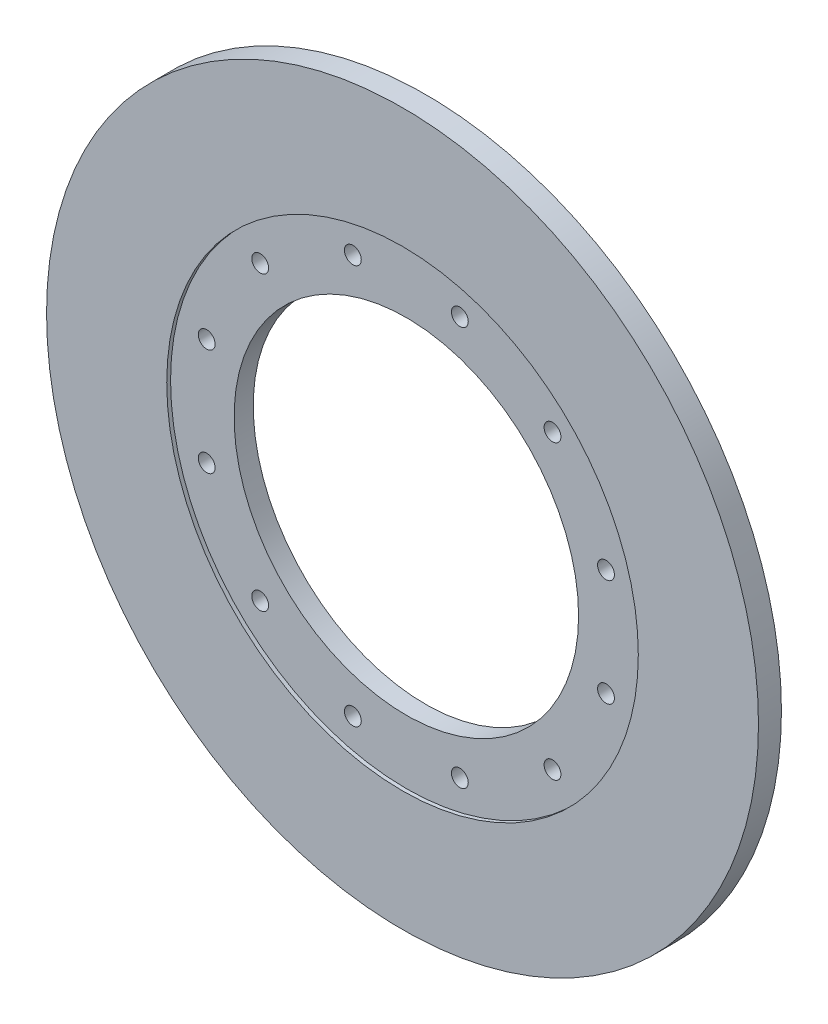
from build123d import *

# Parameters (mm, degrees)
SKETCH1_R               = 465
SKETCH1_R_2             = 225
BOSS_EXTRUDE1_DEPTH     = 30
SKETCH2_R               = 308
CUT_EXTRUDE1_DEPTH      = 5
CUT_EXTRUDE7_DEPTH      = 659.293247725
CUT_EXTRUDE7_DEPTH_BACK = 659.293247725
SKETCH4_R               = 11


with BuildPart() as part:
    # Sketch1 → Boss-Extrude1 (new body)
    with BuildSketch(Plane.XY):
        Circle(SKETCH1_R)
        Circle(SKETCH1_R_2, mode=Mode.SUBTRACT)
    extrude(amount=BOSS_EXTRUDE1_DEPTH)

    # Sketch2 → Cut-Extrude1 (cut)
    with BuildSketch(Plane.XY.offset(30)):
        Circle(SKETCH2_R)
    extrude(amount=-CUT_EXTRUDE1_DEPTH, mode=Mode.SUBTRACT)

    # Sketch4 → Cut-Extrude7 (cut, two sides: drawn at the far end of the back side and taken through both)
    with BuildSketch(Plane(origin=(0, 0, 0), x_dir=(-1, 0, 0), z_dir=(0, 0, -1)).offset(-CUT_EXTRUDE7_DEPTH_BACK)):
        with Locations(Location((-260.799973098, 69.881142178, 0), (0, 0, 180))):
            Circle(SKETCH4_R)
        with Locations(Location((-190.91883092, 190.91883092, 0), (0, 0, 180))):
            Circle(SKETCH4_R)
        with Locations(Location((-69.881142178, 260.799973098, 0), (0, 0, 180))):
            Circle(SKETCH4_R)
        with Locations(Location((69.881142178, 260.799973098, 0), (0, 0, 180))):
            Circle(SKETCH4_R)
        with Locations(Location((190.91883092, 190.91883092, 0), (0, 0, 180))):
            Circle(SKETCH4_R)
        with Locations(Location((260.799973098, 69.881142178, 0), (0, 0, 180))):
            Circle(SKETCH4_R)
        with Locations(Location((260.799973098, -69.881142178, 0), (0, 0, 180))):
            Circle(SKETCH4_R)
        with Locations(Location((190.91883092, -190.91883092, 0), (0, 0, 180))):
            Circle(SKETCH4_R)
        with Locations(Location((69.881142178, -260.799973098, 0), (0, 0, 180))):
            Circle(SKETCH4_R)
        with Locations(Location((-69.881142178, -260.799973098, 0), (0, 0, 180))):
            Circle(SKETCH4_R)
        with Locations(Location((-190.91883092, -190.91883092, 0), (0, 0, 180))):
            Circle(SKETCH4_R)
        with Locations(Location((-260.799973098, -69.881142178, 0), (0, 0, 180))):
            Circle(SKETCH4_R)
    extrude(amount=CUT_EXTRUDE7_DEPTH + CUT_EXTRUDE7_DEPTH_BACK, mode=Mode.SUBTRACT)


solid = part.part
